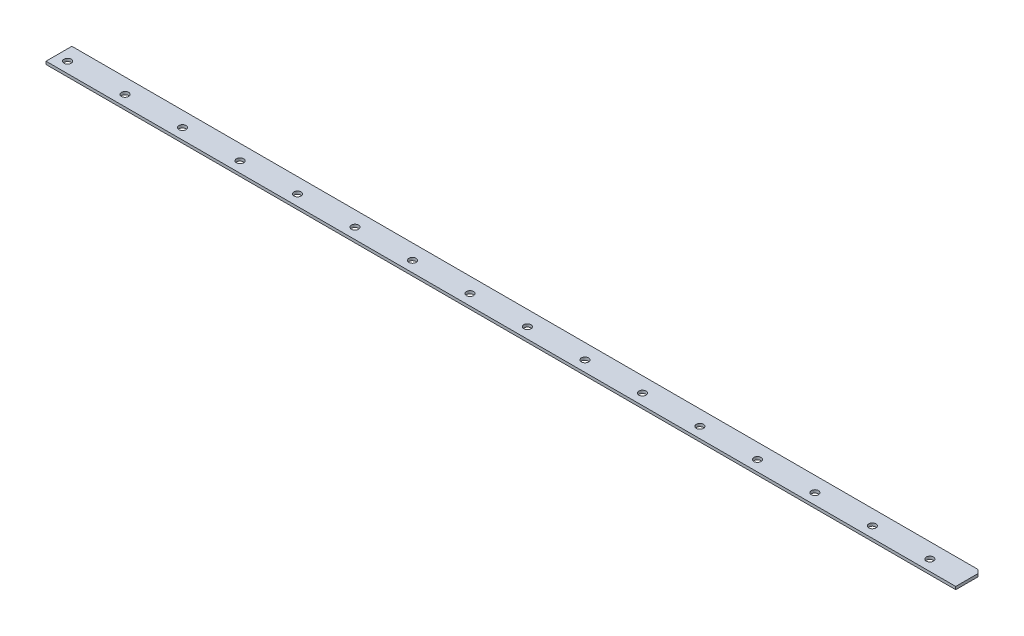
from build123d import *

# Parameters (mm, degrees)
SKETCH_1_W              = 1266
SKETCH_1_H              = 36
EXTRUDE_1_DEPTH         = 4
CHAMFER_1_SIZE          = 5
HOLE_WIZARD_10_0_10_1_D = 10
PATTERN_LINEAR_1_COUNT  = 16
PATTERN_LINEAR_1_PITCH  = 80


with BuildPart() as part:
    # 草图1 → 凸台-拉伸1 (new body)
    with BuildSketch(Plane(origin=(0, 0, 0), x_dir=(1, 0, 0), z_dir=(0, 1, 0))):
        with Locations((-633, -18)):
            Rectangle(SKETCH_1_W, SKETCH_1_H)
    extrude(amount=EXTRUDE_1_DEPTH)

    # 倒角1
    chamfer_1_edges = [part.edges().sort_by_distance(p)[0] for p in [
        (0, 2, 0),
    ]]
    chamfer(chamfer_1_edges, length=CHAMFER_1_SIZE)

    # Ø10.0 (10) 直径孔1 (through all)
    with Locations(Plane(origin=(0, 4, 0), x_dir=(-1, 0, 0), z_dir=(0, 1, 0))):
        with Locations((1251, 21)):
            hole_wizard_10_0_10_1 = Hole(HOLE_WIZARD_10_0_10_1_D / 2)

    # 阵列(线性)1: Ø10.0 (10) 直径孔1 ×16
    with Locations(*[(i * PATTERN_LINEAR_1_PITCH, 0, 0) for i in range(1, PATTERN_LINEAR_1_COUNT)]):
        add(hole_wizard_10_0_10_1, mode=Mode.SUBTRACT)


solid = part.part
